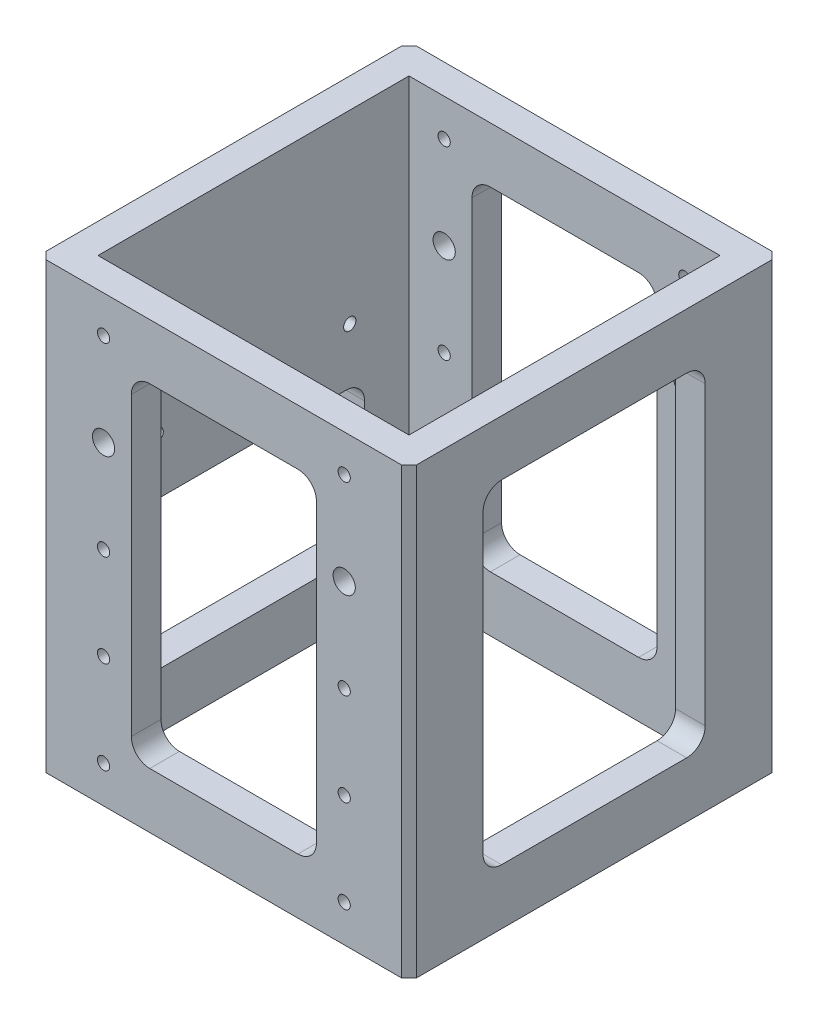
from build123d import *

# Parameters (mm, degrees)
BOSS_EXTRUDE1_DEPTH        = 120
SKETCH3_W                  = 8
SKETCH3_H                  = 100
BOSS_EXTRUDE2_DEPTH        = 120
SKETCH4_W                  = 84
SKETCH4_H                  = 84
CUT_EXTRUDE2_DEPTH         = 140.283882772
SKETCH6_R                  = 1.034396221
SKETCH6_R_2                = 1
CUT_EXTRUDE4_DEPTH         = 7
M4_TAPPED_HOLE1_AT_2_COUNT = 2
M4_TAPPED_HOLE1_AT_2_PITCH = 65
M4_TAPPED_HOLE1_AT_3_COUNT = 2
M4_TAPPED_HOLE1_AT_3_PITCH = 119.268604419
M4_TAPPED_HOLE1_AT_4_COUNT = 2
M4_TAPPED_HOLE1_AT_4_PITCH = 100
M4_TAPPED_HOLE1_AT_5_COUNT = 2
M4_TAPPED_HOLE1_AT_5_PITCH = 50
M4_TAPPED_HOLE1_AT_6_COUNT = 2
M4_TAPPED_HOLE1_AT_6_PITCH = 82.006097334
M4_TAPPED_HOLE2_D          = 3.3
M4_TAPPED_HOLE2_DEPTH      = 11.5
M4_TAPPED_HOLE2_TIP        = 0.991420021
F_6_0_6_DIAMETER_HOLE1_D   = 6
CUT_EXTRUDE5_DEPTH         = 165.012194669
CUT_EXTRUDE6_REACH         = 166.012
CUT_EXTRUDE7_REACH         = 166.012
M4_TAPPED_HOLE3_REACH      = 166.012
M4_TAPPED_HOLE3_BORE_R     = 1.65
CHAMFER1_SIZE              = 2


with BuildPart() as part:
    # Sketch1 → Boss-Extrude1 (new body)
    with BuildSketch(Plane(origin=(0, 0, 0), x_dir=(1, 0, 0), z_dir=(0, 1, 0))):
        Polygon((-42, 50), (42, 50), (42, 42), (3, 42), (3, -42), (42, -42), (42, -50), (-42, -50), (-42, -42), (-3, -42), (-3, 42), (-42, 42), align=None)
    extrude(amount=BOSS_EXTRUDE1_DEPTH)

    # Sketch3 → Boss-Extrude2 (add)
    with BuildSketch(Plane(origin=(0, 120, 0), x_dir=(1, 0, 0), z_dir=(0, 1, 0))):
        with Locations((-46, 0)):
            Rectangle(SKETCH3_W, SKETCH3_H)
        with Locations((46, 0)):
            Rectangle(SKETCH3_W, SKETCH3_H)
    extrude(amount=-BOSS_EXTRUDE2_DEPTH)

    # Sketch4 → Cut-Extrude2 (cut, through all)
    with BuildSketch(Plane(origin=(0, 120, 0), x_dir=(1, 0, 0), z_dir=(0, 1, 0))):
        Rectangle(SKETCH4_W, SKETCH4_H)
    extrude(amount=-CUT_EXTRUDE2_DEPTH, mode=Mode.SUBTRACT)

    # Sketch6 → Cut-Extrude4 (cut)
    with BuildSketch(Plane.XY.offset(50)):
        with Locations((-32.5, 60)):
            Circle(SKETCH6_R)
        with Locations(Location((32.5, 60, 0), (0, 0, 180))):
            Circle(SKETCH6_R)
        with Locations((-32.5, 110)):
            Circle(SKETCH6_R_2)
        with Locations(Location((32.5, 110, 0), (0, 0, 180))):
            Circle(SKETCH6_R_2)
        with Locations((32.5, 10)):
            Circle(SKETCH6_R_2)
        with Locations(Location((-32.5, 10, 0), (0, 0, 180))):
            Circle(SKETCH6_R_2)
    extrude(amount=-CUT_EXTRUDE4_DEPTH, mode=Mode.SUBTRACT)

    # Sketch7 → M4 Tapped Hole1 (revolve, cut)
    with BuildSketch(Plane(origin=(-32.5, 110, 50), x_dir=(0, -1, 0), z_dir=(1, 0, 0))):
        Polygon((0, 0), (0, 11.091420021), (1.65, 10.1), (1.65, 0), align=None)
    m4_tapped_hole1 = revolve(axis=Axis((-32.5, 110, 56.35), (0, 0, -1)), mode=Mode.SUBTRACT)

    # M4 Tapped Hole1 at 2: M4 Tapped Hole1 ×2
    with Locations(*[(i * M4_TAPPED_HOLE1_AT_2_PITCH, 0, 0) for i in range(1, M4_TAPPED_HOLE1_AT_2_COUNT)]):
        add(m4_tapped_hole1, mode=Mode.SUBTRACT)

    # M4 Tapped Hole1 at 3: M4 Tapped Hole1 ×2
    with Locations(*[Vector(0.5449883505954143, -0.8384436163006371, 0) * (i * M4_TAPPED_HOLE1_AT_3_PITCH) for i in range(1, M4_TAPPED_HOLE1_AT_3_COUNT)]):
        add(m4_tapped_hole1, mode=Mode.SUBTRACT)

    # M4 Tapped Hole1 at 4: M4 Tapped Hole1 ×2
    with Locations(*[(0, -i * M4_TAPPED_HOLE1_AT_4_PITCH, 0) for i in range(1, M4_TAPPED_HOLE1_AT_4_COUNT)]):
        add(m4_tapped_hole1, mode=Mode.SUBTRACT)

    # M4 Tapped Hole1 at 5: M4 Tapped Hole1 ×2
    with Locations(*[(0, -i * M4_TAPPED_HOLE1_AT_5_PITCH, 0) for i in range(1, M4_TAPPED_HOLE1_AT_5_COUNT)]):
        add(m4_tapped_hole1, mode=Mode.SUBTRACT)

    # M4 Tapped Hole1 at 6: M4 Tapped Hole1 ×2
    with Locations(*[Vector(0.7926239891046003, -0.6097107608496921, 0) * (i * M4_TAPPED_HOLE1_AT_6_PITCH) for i in range(1, M4_TAPPED_HOLE1_AT_6_COUNT)]):
        add(m4_tapped_hole1, mode=Mode.SUBTRACT)

    # Mirror2: M4 Tapped Hole1 across plane
    add(m4_tapped_hole1.mirror(Plane.XY), mode=Mode.SUBTRACT)

    # Mirror2 copy 1 sketch → Mirror2 copy 1 (revolve, cut)
    with BuildSketch(Plane(origin=(32.5, 110, -50), x_dir=(0, -1, 0), z_dir=(1, 0, 0))):
        Polygon((0, 0), (0, -11.091420021), (1.65, -10.1), (1.65, 0), align=None)
    revolve(axis=Axis((32.5, 110, -56.35), (0, 0, -1)), mode=Mode.SUBTRACT)

    # Mirror2 copy 2 sketch → Mirror2 copy 2 (revolve, cut)
    with BuildSketch(Plane(origin=(32.5, 10, -50), x_dir=(0, -1, 0), z_dir=(1, 0, 0))):
        Polygon((0, 0), (0, -11.091420021), (1.65, -10.1), (1.65, 0), align=None)
    revolve(axis=Axis((32.5, 10, -56.35), (0, 0, -1)), mode=Mode.SUBTRACT)

    # Mirror2 copy 3 sketch → Mirror2 copy 3 (revolve, cut)
    with BuildSketch(Plane(origin=(-32.5, 10, -50), x_dir=(0, -1, 0), z_dir=(1, 0, 0))):
        Polygon((0, 0), (0, -11.091420021), (1.65, -10.1), (1.65, 0), align=None)
    revolve(axis=Axis((-32.5, 10, -56.35), (0, 0, -1)), mode=Mode.SUBTRACT)

    # Mirror2 copy 4 sketch → Mirror2 copy 4 (revolve, cut)
    with BuildSketch(Plane(origin=(-32.5, 60, -50), x_dir=(0, -1, 0), z_dir=(1, 0, 0))):
        Polygon((0, 0), (0, -11.091420021), (1.65, -10.1), (1.65, 0), align=None)
    revolve(axis=Axis((-32.5, 60, -56.35), (0, 0, -1)), mode=Mode.SUBTRACT)

    # Mirror2 copy 5 sketch → Mirror2 copy 5 (revolve, cut)
    with BuildSketch(Plane(origin=(32.5, 60, -50), x_dir=(0, -1, 0), z_dir=(1, 0, 0))):
        Polygon((0, 0), (0, -11.091420021), (1.65, -10.1), (1.65, 0), align=None)
    revolve(axis=Axis((32.5, 60, -56.35), (0, 0, -1)), mode=Mode.SUBTRACT)

    # M4 Tapped Hole2
    with Locations(Plane.ZY.offset(50)):
        with Locations((-26, 70), (26, 70), (37, 70)):
            Hole(M4_TAPPED_HOLE2_D / 2, depth=M4_TAPPED_HOLE2_DEPTH)
            with Locations((0, 0, -(M4_TAPPED_HOLE2_DEPTH + M4_TAPPED_HOLE2_TIP / 2))):  # 118° drill point
                Cone(0, M4_TAPPED_HOLE2_D / 2, M4_TAPPED_HOLE2_TIP, mode=Mode.SUBTRACT)

    # Ø6.0 (6) Diameter Hole1 (through all)
    with Locations(Plane.XY.offset(50)):
        with Locations((-32.5, 85), (32.5, 85)):
            Hole(F_6_0_6_DIAMETER_HOLE1_D / 2)

    # Sketch12 → Cut-Extrude5 (cut, through all)
    with BuildSketch(Plane.XY.offset(50)):
        with BuildLine():
            Line((-20, 105), (20, 105))
            ThreePointArc((20, 105), (23.535533906, 103.535533906), (25, 100))
            Line((25, 100), (25, 20))
            ThreePointArc((25, 20), (23.535533906, 16.464466094), (20, 15))
            Line((20, 15), (-20, 15))
            ThreePointArc((-20, 15), (-23.535533906, 16.464466094), (-25, 20))
            Line((-25, 20), (-25, 100))
            ThreePointArc((-25, 100), (-23.535533906, 103.535533906), (-20, 105))
        make_face()
    extrude(amount=-CUT_EXTRUDE5_DEPTH, mode=Mode.SUBTRACT)

    # Sketch13 → Cut-Extrude6 (cut, up to next)
    with BuildSketch(Plane(origin=(50, 0, 0), x_dir=(0, 0, -1), z_dir=(1, 0, 0)), mode=Mode.PRIVATE) as cut_extrude6_sk1:
        with BuildLine():
            Line((-25, 105), (25, 105))
            ThreePointArc((25, 105), (28.535533906, 103.535533906), (30, 100))
            Line((30, 100), (30, 20))
            ThreePointArc((30, 20), (28.535533906, 16.464466094), (25, 15))
            Line((25, 15), (-25, 15))
            ThreePointArc((-25, 15), (-28.535533906, 16.464466094), (-30, 20))
            Line((-30, 20), (-30, 100))
            ThreePointArc((-30, 100), (-28.535533906, 103.535533906), (-25, 105))
        make_face()
    cut_extrude6_tool1 = extrude(cut_extrude6_sk1.sketch, amount=-CUT_EXTRUDE6_REACH, mode=Mode.PRIVATE) & part.part
    add(cut_extrude6_tool1.solids().sort_by_distance((50, 60, 0))[0], mode=Mode.SUBTRACT)

    # Sketch14 → Cut-Extrude7 (cut, up to next)
    with BuildSketch(Plane.ZY.offset(50), mode=Mode.PRIVATE) as cut_extrude7_sk1:
        with BuildLine():
            Line((-25, 55), (25, 55))
            ThreePointArc((25, 55), (28.535533906, 53.535533906), (30, 50))
            Line((30, 50), (30, 20))
            ThreePointArc((30, 20), (28.535533906, 16.464466094), (25, 15))
            Line((25, 15), (-25, 15))
            ThreePointArc((-25, 15), (-28.535533906, 16.464466094), (-30, 20))
            Line((-30, 20), (-30, 50))
            ThreePointArc((-30, 50), (-28.535533906, 53.535533906), (-25, 55))
        make_face()
    cut_extrude7_tool1 = extrude(cut_extrude7_sk1.sketch, amount=-CUT_EXTRUDE7_REACH, mode=Mode.PRIVATE) & part.part
    add(cut_extrude7_tool1.solids().sort_by_distance((-50, 35, 0))[0], mode=Mode.SUBTRACT)

    # M4 Tapped Hole3 bore → M4 Tapped Hole3 (cut, up to next)
    with BuildSketch(Plane.XY.offset(50), mode=Mode.PRIVATE) as m4_tapped_hole3_sk1:
        with Locations((-32.5, 35)):
            Circle(M4_TAPPED_HOLE3_BORE_R)
    m4_tapped_hole3_tool1 = extrude(m4_tapped_hole3_sk1.sketch, amount=-M4_TAPPED_HOLE3_REACH, mode=Mode.PRIVATE) & part.part
    # M4 Tapped Hole3 bore → M4 Tapped Hole3 (cut, up to next)
    with BuildSketch(Plane.XY.offset(50), mode=Mode.PRIVATE) as m4_tapped_hole3_sk2:
        with Locations((32.5, 35)):
            Circle(M4_TAPPED_HOLE3_BORE_R)
    m4_tapped_hole3_tool2 = extrude(m4_tapped_hole3_sk2.sketch, amount=-M4_TAPPED_HOLE3_REACH, mode=Mode.PRIVATE) & part.part
    m4_tapped_hole3_1 = m4_tapped_hole3_tool1.solids().sort_by_distance((-32.5, 35, 50))[0]
    add(m4_tapped_hole3_1, mode=Mode.SUBTRACT)
    m4_tapped_hole3_2 = m4_tapped_hole3_tool2.solids().sort_by_distance((32.5, 35, 50))[0]
    add(m4_tapped_hole3_2, mode=Mode.SUBTRACT)
    m4_tapped_hole3 = m4_tapped_hole3_1 + m4_tapped_hole3_2  # M4 Tapped Hole3 as one shape, for the pattern or mirror that repeats it

    # Mirror3: M4 Tapped Hole3 across plane
    add(m4_tapped_hole3.mirror(Plane.XY), mode=Mode.SUBTRACT)

    # Chamfer1
    chamfer1_edges = [part.edges().sort_by_distance(p)[0] for p in [
        (-50, 60, 50),
        (-50, 60, -50),
        (50, 60, -50),
        (50, 60, 50),
    ]]
    chamfer(chamfer1_edges, length=CHAMFER1_SIZE)


solid = part.part
